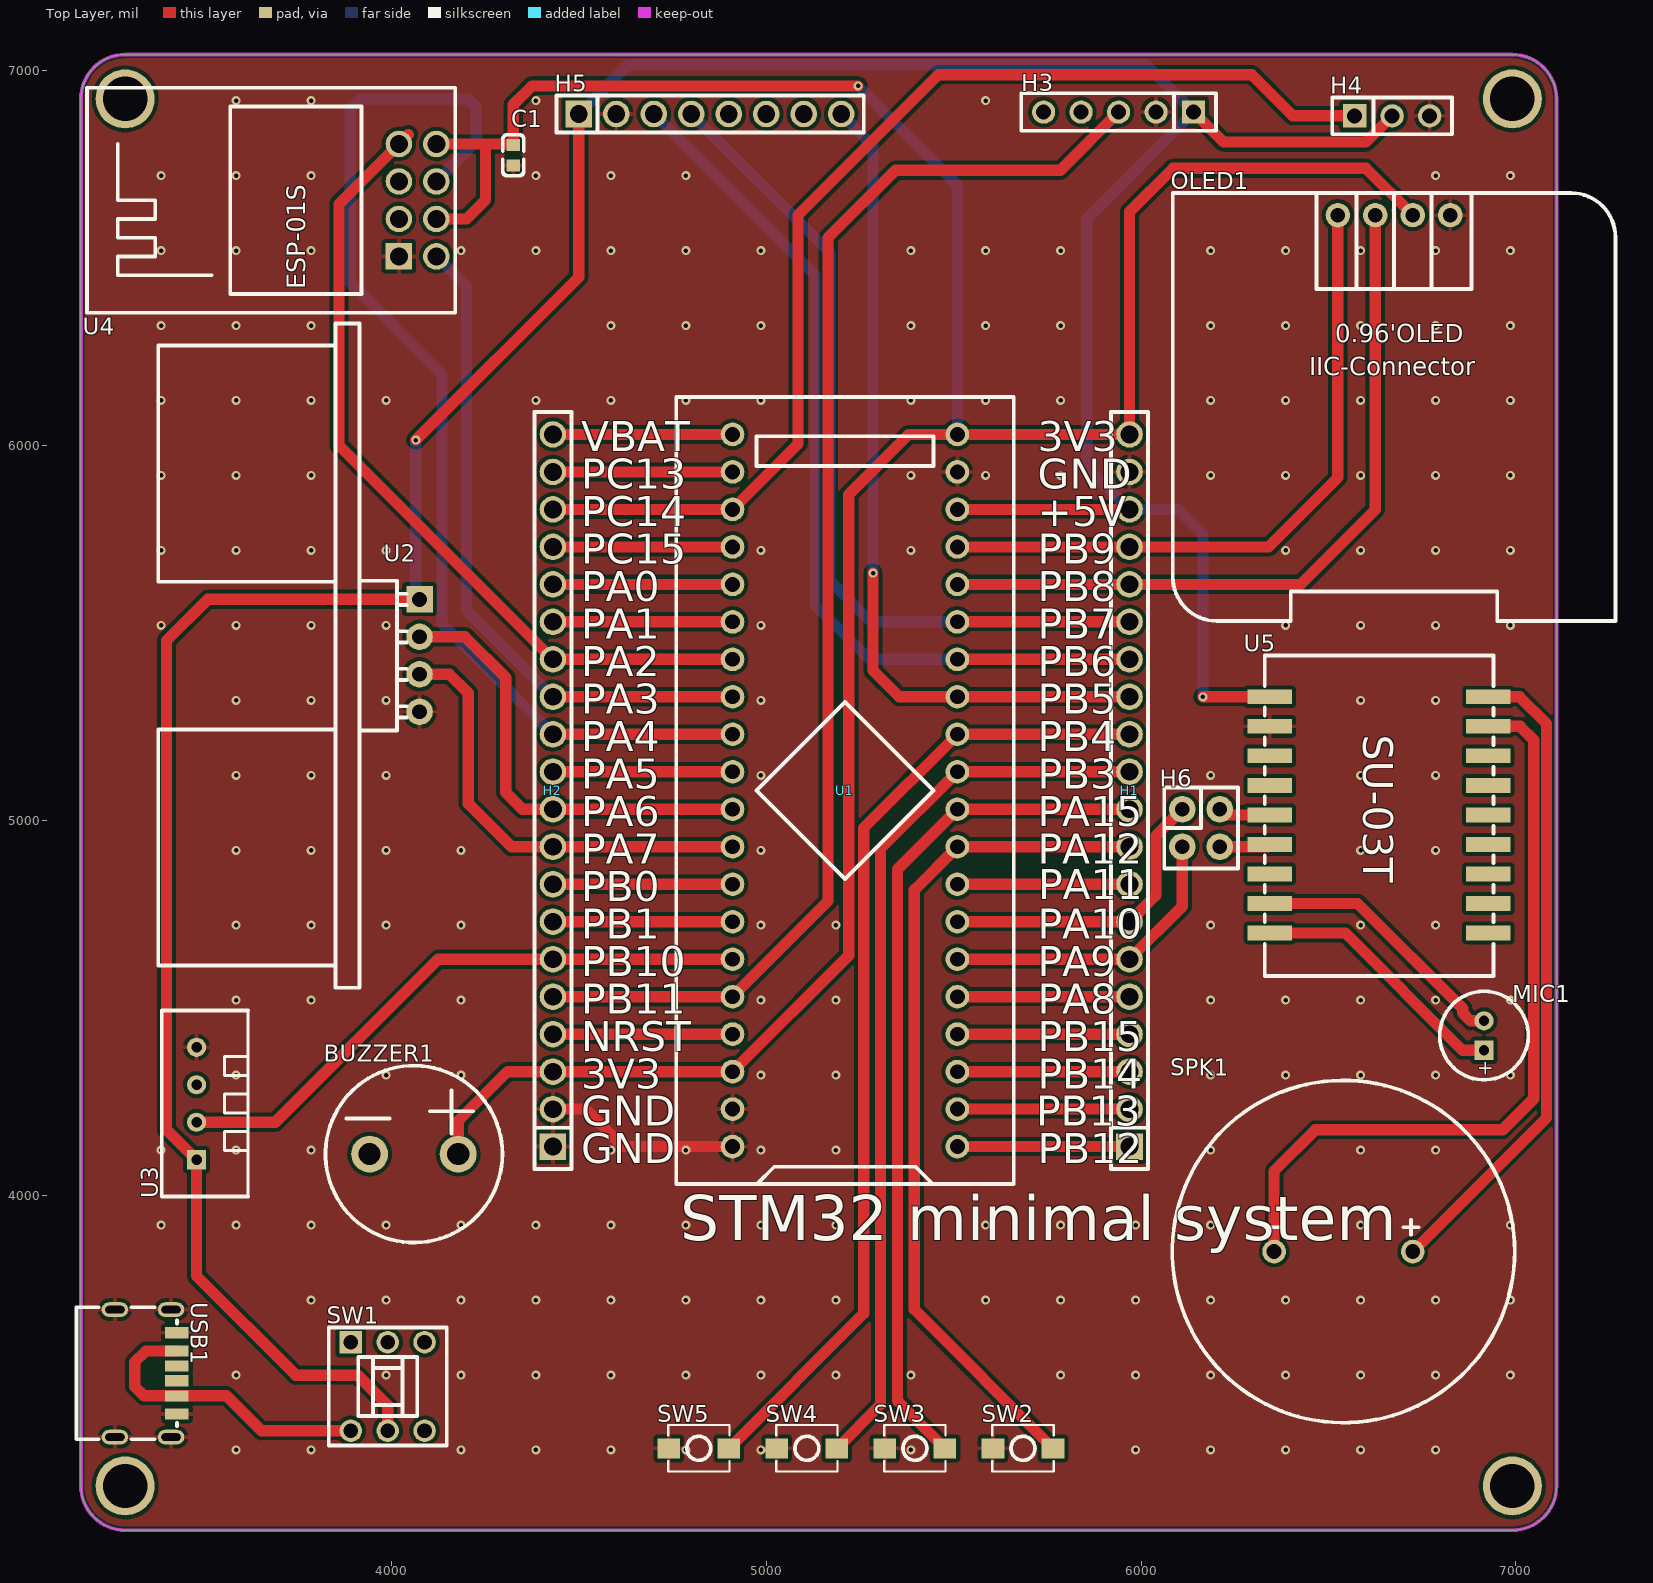
[diagram p0: Top Layer view]
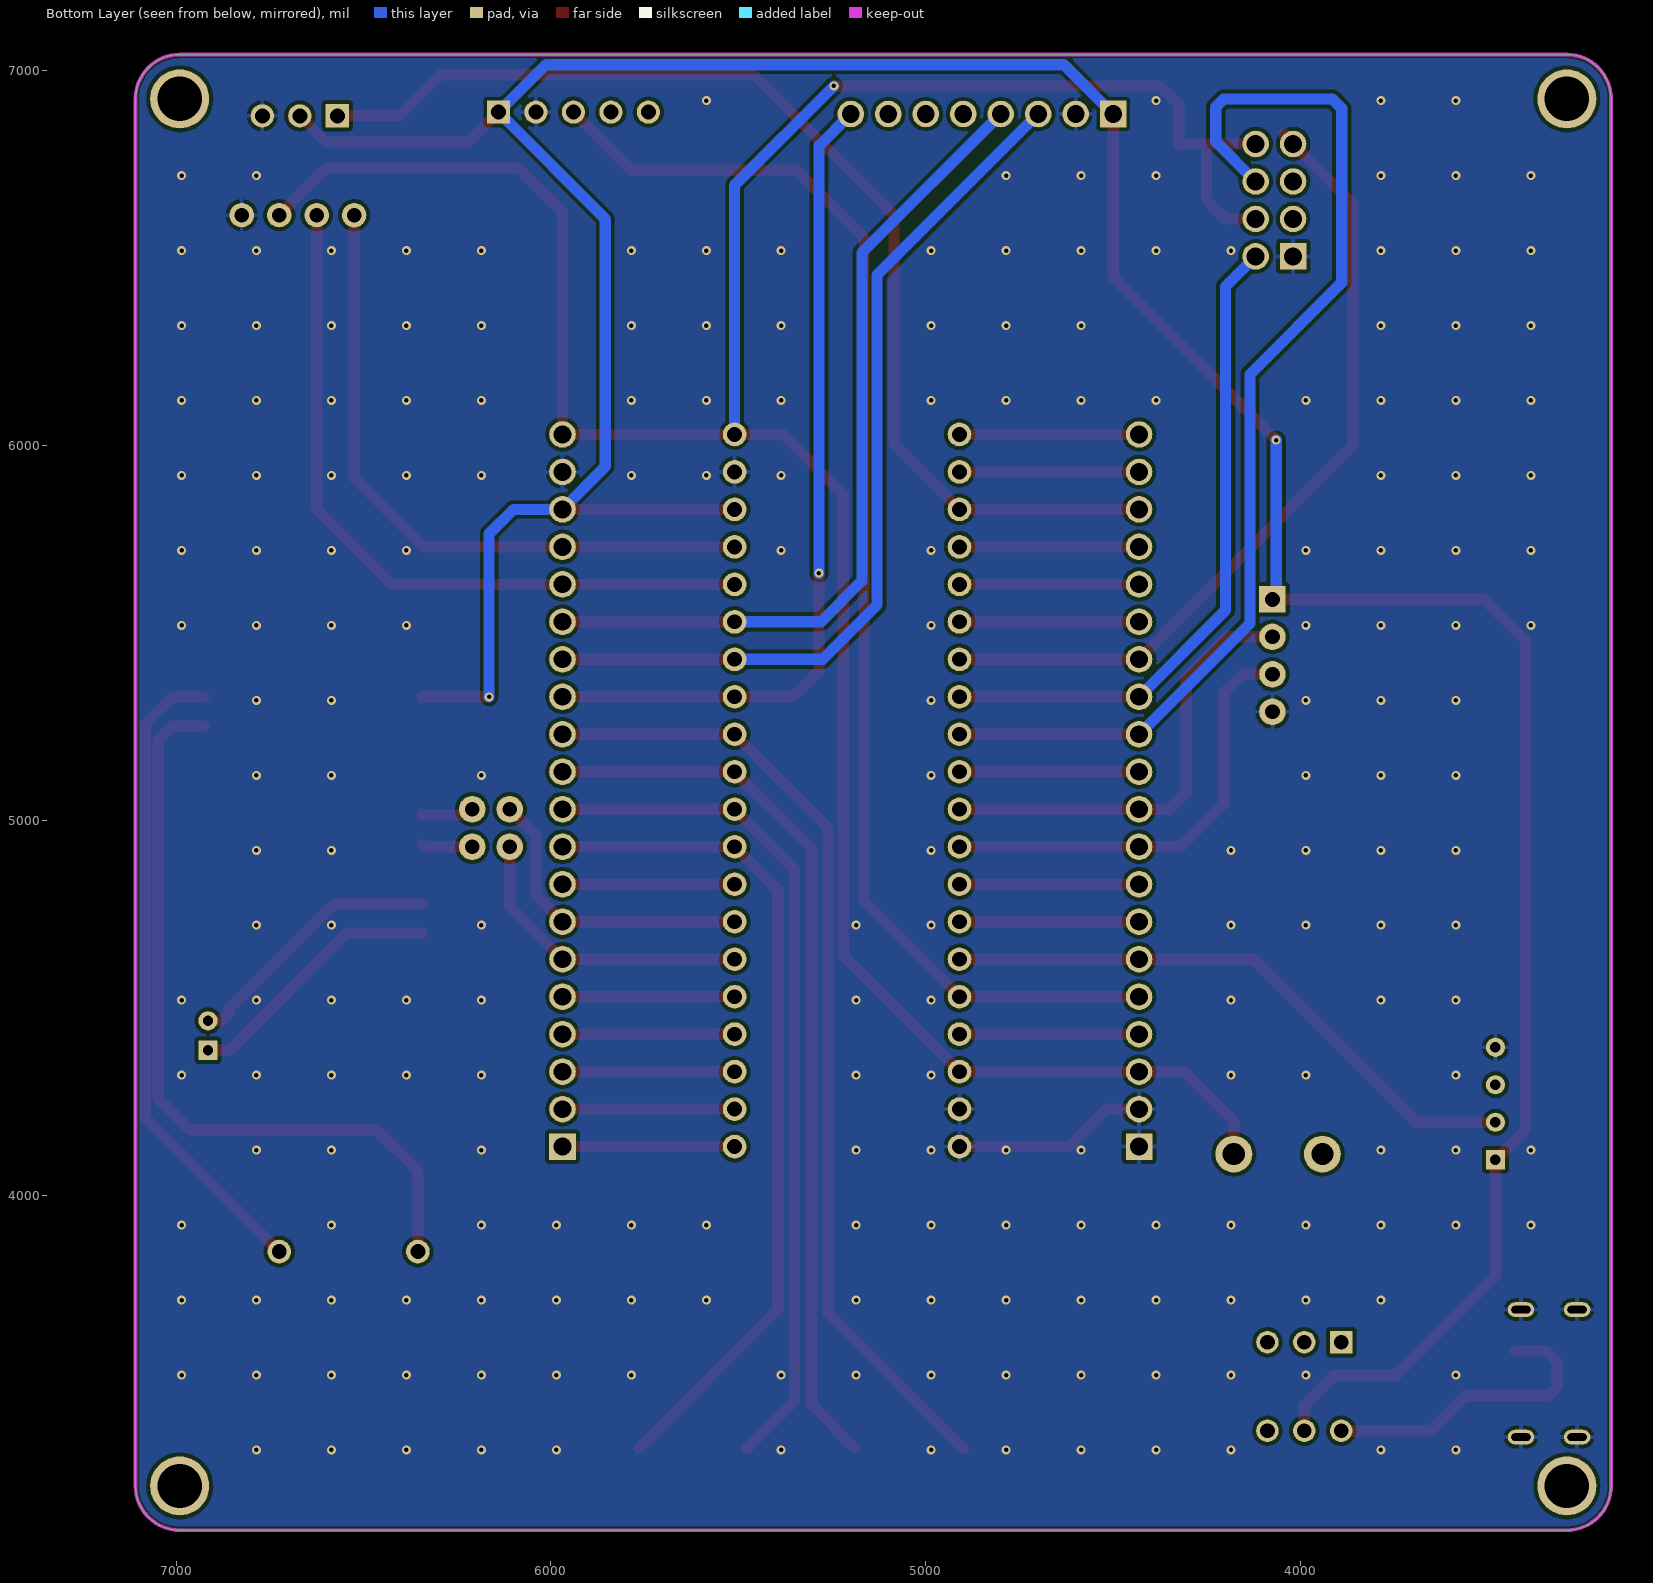
[diagram p1: Bottom Layer view, seen from below]
# Altium PCB MISC89046.pcbdoc
Units mil, origin at the board's own origin, x right, y up, seen from the top; angles counter-clockwise.
Board outline 3937.01 x 3937.01 mil, 2 copper layers (Top Layer, Bottom Layer), stack 62.206 mil thick; 22 components, 45 nets, 174 pads, 212 vias.

## Layer stack, top to bottom
Top Solder Mask Layer: solder mask 0.394, Dk 3.3
Top Layer: signal copper 1.379
Dielectric1: surface 59.449, FR4, Dk 4.5
Bottom Layer: signal copper 1.378
Bottom Solder Mask Layer: solder mask 0.394, Dk 3.3

## Board outline
3289.61,7043.5 ccw(c3289.61,6925.39) 3171.5,6925.39 3171.5,3224.61 ccw(c3289.61,3224.61) 3289.61,3106.5 6990.39,3106.5 ccw(c6990.39,3224.61) 7108.5,3224.61 7108.5,6925.39 ccw(c6990.39,6925.39) 6990.39,7043.5 3289.61,7043.5

## Design rules (kind name [scope] priority, off if disabled: settings)
BoardOutlineClearance copperThickness2oz_1 [All] p2 off: genericclearance=7.99 ignorepadtopadclearanceinfootprint=FALSE except(0: Arc-SplitContinuation Track-SplitContinuation SMDPad-SplitContinuation THPad-SplitContinuation Via-SplitContinuation Fill-SplitContinuation Region-SplitContinuation Poly-SplitContinuation Text-SplitContinuation Hole-SplitContinuation; 5.98: Arc-CutoutEdge Track-CutoutEdge SMDPad-CutoutEdge THPad-CutoutEdge Via-CutoutEdge Text-CutoutEdge; 6.9: Hole-OutlineEdge Hole-CutoutEdge; 10: Poly-OutlineEdge Poly-CutoutEdge; 11.81: Arc-OutlineEdge Track-OutlineEdge SMDPad-OutlineEdge THPad-OutlineEdge Via-OutlineEdge Fill-OutlineEdge Region-OutlineEdge Text-OutlineEdge Fill-CutoutEdge Region-CutoutEdge)
BoardOutlineClearance Plane_innerPlane_1 [All] p4 off: genericclearance=4.02 ignorepadtopadclearanceinfootprint=FALSE except(0: Arc-SplitContinuation Track-SplitContinuation SMDPad-SplitContinuation THPad-SplitContinuation Via-SplitContinuation Fill-SplitContinuation Region-SplitContinuation Poly-SplitContinuation Text-SplitContinuation Hole-SplitContinuation; 5.98: Arc-CutoutEdge Track-CutoutEdge SMDPad-CutoutEdge THPad-CutoutEdge Via-CutoutEdge Text-CutoutEdge; 6.9: Hole-OutlineEdge Hole-CutoutEdge; 10: Poly-OutlineEdge Poly-CutoutEdge; 11.81: Arc-OutlineEdge Track-OutlineEdge SMDPad-OutlineEdge THPad-OutlineEdge Via-OutlineEdge Fill-OutlineEdge Region-OutlineEdge Text-OutlineEdge Fill-CutoutEdge Region-CutoutEdge)
BoardOutlineClearance Copper_copperRegion_1 [All] p6 off: genericclearance=4.02 ignorepadtopadclearanceinfootprint=FALSE except(0: Arc-SplitContinuation Track-SplitContinuation SMDPad-SplitContinuation THPad-SplitContinuation Via-SplitContinuation Fill-SplitContinuation Region-SplitContinuation Poly-SplitContinuation Text-SplitContinuation Hole-SplitContinuation; 5.98: Arc-CutoutEdge Track-CutoutEdge SMDPad-CutoutEdge THPad-CutoutEdge Via-CutoutEdge Text-CutoutEdge; 6.9: Hole-OutlineEdge Hole-CutoutEdge; 10: Poly-OutlineEdge Poly-CutoutEdge; 11.81: Arc-OutlineEdge Track-OutlineEdge SMDPad-OutlineEdge THPad-OutlineEdge Via-OutlineEdge Fill-OutlineEdge Region-OutlineEdge Text-OutlineEdge Fill-CutoutEdge Region-CutoutEdge)
BoardOutlineClearance copperThickness1oz_1 [All] p8: genericclearance=4.02 ignorepadtopadclearanceinfootprint=FALSE except(0: Arc-SplitContinuation Track-SplitContinuation SMDPad-SplitContinuation THPad-SplitContinuation Via-SplitContinuation Fill-SplitContinuation Region-SplitContinuation Poly-SplitContinuation Text-SplitContinuation Hole-SplitContinuation; 5.98: Arc-CutoutEdge Track-CutoutEdge SMDPad-CutoutEdge THPad-CutoutEdge Via-CutoutEdge Text-CutoutEdge; 6.9: Hole-OutlineEdge Hole-CutoutEdge; 10: Poly-OutlineEdge Poly-CutoutEdge; 11.81: Arc-OutlineEdge Track-OutlineEdge SMDPad-OutlineEdge THPad-OutlineEdge Via-OutlineEdge Fill-OutlineEdge Region-OutlineEdge Text-OutlineEdge Fill-CutoutEdge Region-CutoutEdge)
Clearance copperThickness2oz [All] p1 off: gap=7.99 ignorepadtopadclearanceinfootprint=FALSE except(5.98: SMDPad-Track SMDPad-SMDPad THPad-Track SMDPad-THPad THPad-THPad Track-Via SMDPad-Via THPad-Via Via-Via Fill-SMDPad Region-SMDPad Fill-THPad Region-THPad Fill-Via Region-Via Fill-Fill Fill-Region Region-Region Arc-Track Arc-SMDPad Arc-THPad Arc-Via Fill-Arc Region-Arc Arc-Arc Text-Track SMDPad-Text Text-THPad Text-Via Fill-Text Region-Text Arc-Text Text-Text; 6.9: Hole-Track Hole-SMDPad Hole-THPad Hole-Via Fill-Hole Region-Hole Hole-Arc Hole-Text; 10: Poly-Track Poly-SMDPad Poly-THPad Poly-Via Poly-Fill Poly-Region Poly-Poly Poly-Arc Poly-Text Poly-Hole; 11.81: Fill-Track Region-Track)
Clearance Plane_innerPlane [All] p3 off: gap=4.02 ignorepadtopadclearanceinfootprint=FALSE except(5.98: SMDPad-Track SMDPad-SMDPad THPad-Track SMDPad-THPad THPad-THPad Track-Via SMDPad-Via THPad-Via Via-Via Fill-SMDPad Region-SMDPad Fill-THPad Region-THPad Fill-Via Region-Via Fill-Fill Fill-Region Region-Region Arc-Track Arc-SMDPad Arc-THPad Arc-Via Fill-Arc Region-Arc Arc-Arc Text-Track SMDPad-Text Text-THPad Text-Via Fill-Text Region-Text Arc-Text Text-Text; 6.9: Hole-Track Hole-SMDPad Hole-THPad Hole-Via Fill-Hole Region-Hole Hole-Arc Hole-Text; 10: Poly-Track Poly-SMDPad Poly-THPad Poly-Via Poly-Fill Poly-Region Poly-Poly Poly-Arc Poly-Text Poly-Hole; 11.81: Fill-Track Region-Track)
Clearance Copper_copperRegion [All] p5 off: gap=4.02 ignorepadtopadclearanceinfootprint=FALSE except(5.98: SMDPad-Track SMDPad-SMDPad THPad-Track SMDPad-THPad THPad-THPad Track-Via SMDPad-Via THPad-Via Via-Via Fill-SMDPad Region-SMDPad Fill-THPad Region-THPad Fill-Via Region-Via Fill-Fill Fill-Region Region-Region Arc-Track Arc-SMDPad Arc-THPad Arc-Via Fill-Arc Region-Arc Arc-Arc Text-Track SMDPad-Text Text-THPad Text-Via Fill-Text Region-Text Arc-Text Text-Text; 6.9: Hole-Track Hole-SMDPad Hole-THPad Hole-Via Fill-Hole Region-Hole Hole-Arc Hole-Text; 10: Poly-Track Poly-SMDPad Poly-THPad Poly-Via Poly-Fill Poly-Region Poly-Poly Poly-Arc Poly-Text Poly-Hole; 11.81: Fill-Track Region-Track)
Clearance copperThickness1oz [All] p7: gap=4.02 ignorepadtopadclearanceinfootprint=FALSE except(5.98: SMDPad-Track SMDPad-SMDPad THPad-Track SMDPad-THPad THPad-THPad Track-Via SMDPad-Via THPad-Via Via-Via Fill-SMDPad Region-SMDPad Fill-THPad Region-THPad Fill-Via Region-Via Fill-Fill Fill-Region Region-Region Arc-Track Arc-SMDPad Arc-THPad Arc-Via Fill-Arc Region-Arc Arc-Arc Text-Track SMDPad-Text Text-THPad Text-Via Fill-Text Region-Text Arc-Text Text-Text; 6.9: Hole-Track Hole-SMDPad Hole-THPad Hole-Via Fill-Hole Region-Hole Hole-Arc Hole-Text; 10: Poly-Track Poly-SMDPad Poly-THPad Poly-Via Poly-Fill Poly-Region Poly-Poly Poly-Arc Poly-Text Poly-Hole; 11.81: Fill-Track Region-Track)
DiffPairsRouting differentialPair [All] p1: maxlimit=6 minlimit=6 mostfreqgap=6 toplayer_minwidth=5 toplayer_prefwidth=10 toplayer_maxwidth=100 toplayer_mingap=6 toplayer_prefgap=6 toplayer_maxgap=6 bottomlayer_minwidth=5 bottomlayer_prefwidth=10 bottomlayer_maxwidth=100 bottomlayer_mingap=6 bottomlayer_prefgap=6 bottomlayer_maxgap=6 maxuncoupledlength=10
HoleToHoleClearance otherClearance [All] p1: gap=11.81 allowstackedmicrovias=TRUE
Length netLength [All] p1: minlimit=0 maxlimit=0
PasteMaskExpansion pasteMaskExpansion [All] p1: expansion=0
PlaneConnect innerPlane [All] p1: planeconnectstyle=Relief reliefexpansion=20 reliefentries=4 reliefconductorwidth=10 reliefairgap=10
PolygonConnect copperRegion [All] p1: connectstyle=Relief reliefconductorwidth=10 reliefentries=4 polygonreliefangle="90 Angle" airgapwidth=10 via.connectstyle=Relief via.reliefconductorwidth=10 via.reliefentries=4 via.polygonreliefangle="90 Angle" via.airgapwidth=10
RoutingVias viaSize [All] p1: holewidth=12.01 width=24.02 viastyle="Through Hole" minholewidth=11.81 minwidth=19.68 maxholewidth=248.03 maxwidth=393.7
SolderMaskExpansion solderMaskExpansion [IsVia] p1: expansion=-1000 istentingtop=TRUE
SolderMaskExpansion solderMaskExpansion [All] p2: expansion=2 istentingtop=FALSE
Width copperThickness2oz_2 [All] p1 off: maxlimit=100 minlimit=8 preferedwidth=10
Width copperThickness1oz_2 [All] p2: maxlimit=100 minlimit=5 preferedwidth=10

## Components (designator, comment, footprint, x,y, rotation, side; value= is the part's Value field where it differs from the comment)
BUZZER1 "Buz" BUZ-TH_BD12.0-P6.00-D0.9-RD 4060,4110 r0 top
C1 "100nF" C0603 4325,6775 r270 top
H1 "" HDR-TH_20P-P2.54-V-F 5969.16,5080 r90 top
H2 "" HDR-TH_20P-P2.54-V-F 4430.95,5080 r90 top
H3 "ATGM336H module" HDR-TH_5P-P2.54-V-F 5940,6890 r180 top
H4 "Vibration module" HDR-TH_3P-P2.54-V-F 6670,6880 r0 top
H5 "MPU6050" HDR-TH_8P-P2.54-V-F-1 4850,6885 r0 top
H6 "" HDR-TH_4P-P2.54-V-F-R2-C2-S2.54 6160,4980 r270 top
MIC1 "MIC" MIC-TH_BD6.0-P2.00 6915,4426.26 r90 top
OLED1 "" 0.96OLED_4P 6675,6615 r0 top
SPK1 "FS-2308" BEEP-TH_BD23.2-P9.20-D1.0 6540,3850 r0 top
SW1 "PS081-06L135D1-JF-G" SW-TH_6P-L8.0-W8.0-P2.50-TL 3990,3490 r0 top
SW2 "" Key_SMD_3x4x2 5685,3325 r0 top
SW3 "" Key_SMD_3x4x2 5396.67,3325 r0 top
SW4 "" Key_SMD_3x4x2 5108.33,3325 r0 top
SW5 "" Key_SMD_3x4x2 4820,3325 r0 top
U1 "STM32F103C8T6-Card" CONN-TH_L53.3-W22.9_STM32F103C8T6-CARD 5210,5080 r90 top
U2 "HC-SR04" TH_HC-SR04V 4075,5440 r270 top
U3 "DHT11 temperature and humidity" SENSOR-TH_DHT11 3480,4245 r90 top
U4 "ESP-01S" WIFIM-TH_ESP-01S 4070,6655 r90 top
U5 "SU-03T" COMM-SMD_18P-L21.0-W15.0-P2.00 6635,5015 r0 top
USB1 "TYPEC-250D-BCP6" USB-C-SMD_TYPEC-250D-BCP6 3345,3525 r270 top

## Footprints (in the part's own frame and the unit in brackets; to place one, negate y for a bottom-side part, rotate by r counter-clockwise, add the part's x,y. Pads: shape width x height; smd on the part's side, far side on the other; paste and mask are expansions set on the pad)
0.96OLED_4P [mm]
  round 1.65 hole 1 copper offset 0,0: 1(-3.81,-0.001) 2(-1.27,0.002) 3(1.27,0.002) 4(3.81,0.002)
  silkscreen extent -15,-27.5 15,1.5
BEEP-TH_BD23.2-P9.20-D1.0 [mm]
  round 1.6 hole 1: 1(4.7,0) 2(-4.7,0)
  silkscreen extent -11.6,-11.6 11.6,11.6
BUZ-TH_BD12.0-P6.00-D0.9-RD [mm]
  round 2.5 hole 1.5 paste+0 mask+0.05: 1(-3,0) 2(3,0)
  silkscreen extent -5.99,-5.99 5.99,5.99
C0603 [mm]
  rect 0.8x0.9 smd: 1(-0.7,0) 2(0.7,0)
  silkscreen extent -1.39,-0.71 1.39,0.71
COMM-SMD_18P-L21.0-W15.0-P2.00 [mm]
  rect 3x1 smd: 1(-7.4,8) 2(-7.4,6) 3(-7.4,4) 4(-7.4,2) 5(-7.4,0) 6(-7.4,-2) 7(-7.4,-4) 8(-7.4,-6) 9(-7.4,-8) 10(7.4,-8) 11(7.4,-6) 12(7.4,-4) 13(7.4,-2) 14(7.4,0) 15(7.4,2) 16(7.4,4) 17(7.4,6) 18(7.4,8)
  silkscreen extent -7.75,-10.92 7.75,10.79
CONN-TH_L53.3-W22.9_STM32F103C8T6-CARD [mm]
  round 1.6 hole 1: 1(-24.13,-7.62) 2(-21.59,-7.62) 3(-19.05,-7.62) 4(-16.51,-7.62) 5(-13.97,-7.62) 6(-11.43,-7.62) 7(-8.89,-7.62) 8(-6.35,-7.62) 9(-3.81,-7.62) 10(-1.27,-7.62) 11(1.27,-7.62) 12(3.81,-7.62) 13(6.35,-7.62) 14(8.89,-7.62) 15(11.43,-7.62) 16(13.97,-7.62) 17(16.51,-7.62) 18(19.05,-7.62) 19(21.59,-7.62) 20(24.13,-7.62) 21(24.13,7.62) 22(21.59,7.62) 23(19.05,7.62) 24(16.51,7.62) 25(13.97,7.62) 26(11.43,7.62) 27(8.89,7.62) 28(6.35,7.62) 29(3.81,7.62) 30(1.27,7.62) 31(-1.27,7.62) 32(-3.81,7.62) 33(-6.35,7.62) 34(-8.89,7.62) 35(-11.43,7.62) 36(-13.97,7.62) 37(-16.51,7.62) 38(-19.05,7.62) 39(-21.59,7.62) 40(-24.13,7.62)
  silkscreen extent -26.67,-11.43 26.67,11.43
HDR-TH_3P-P2.54-V-F [mil]
  rect 62x62 hole 40.16: 1(-100,0)
  round 62 hole 40.16: 2(0,0) 3(100,0)
  silkscreen extent -160,-49 160,49
HDR-TH_4P-P2.54-V-F-R2-C2-S2.54 [mm]
  round 1.8 hole 1: 1(-1.27,-1.27) 2(-1.27,1.27) 3(1.27,-1.27) 4(1.27,1.27)
  silkscreen extent -2.74,-2.5 2.74,2.5
HDR-TH_5P-P2.54-V-F [mil]
  rect 62x62 hole 40.16: 1(-200,0)
  round 62 hole 40.16: 2(-100,0) 3(0,0) 4(100,0) 5(200,0)
  silkscreen extent -260,-50 260,50
HDR-TH_8P-P2.54-V-F-1 [mm]
  rect 1.8x1.8 hole 1.2: 1(-8.89,0)
  round 1.8 hole 1.2: 2(-6.35,0) 3(-3.81,0) 4(-1.27,0) 5(1.27,0) 6(3.81,0) 7(6.35,0) 8(8.89,0)
  silkscreen extent -10.41,-1.25 10.41,1.25
HDR-TH_20P-P2.54-V-F [mm]
  rect 1.8x1.8 hole 1.2: 1(-24.13,0)
  round 1.8 hole 1.2: 2(-21.59,0) 3(-19.05,0) 4(-16.51,0) 5(-13.97,0) 6(-11.43,0) 7(-8.89,0) 8(-6.35,0) 9(-3.81,0) 10(-1.27,0) 11(1.27,0) 12(3.81,0) 13(6.35,0) 14(8.89,0) 15(11.43,0) 16(13.97,0) 17(16.51,0) 18(19.05,0) 19(21.59,0) 20(24.13,0)
  silkscreen extent -25.65,-1.25 25.65,1.25
Key_SMD_3x4x2 [mm]
  rect 1.53x1.36 smd paste+0 mask+0.051: 1(-2.035,0) 2(2.035,0)
  silkscreen extent -2.08,-1.58 2.08,1.58
MIC-TH_BD6.0-P2.00 [mm]
  rect 1.3x1.3 hole 0.7: 1(-1,0)
  round 1.3 hole 0.7: 2(1,0)
  silkscreen extent -3,-3 3,3
SENSOR-TH_DHT11 [mil]
  rect 51x51 hole 28: 1(-150,0)
  round 51 hole 28: 2(-50,0) 3(50,0) 4(150,0)
  silkscreen extent -248,-138 248,93
SW-TH_6P-L8.0-W8.0-P2.50-TL [mil]
  rect 60x60 hole 39.37: 1(-98.43,118.11)
  round 60 hole 39.37: 2(0,118.11) 3(98.42,118.11) 4(-98.43,-118.11) 5(0,-118.11) 6(98.42,-118.11)
  silkscreen extent -157,-157 157,157
TH_HC-SR04V [mm]
  rect 1.8x1.8 hole 1.001: 1(-3.81,0)
  round 1.8 hole 1.001: 2(-1.27,0) 3(1.27,0) 4(3.81,0)
  silkscreen extent -22.5,-17.7 22.5,-0.89
USB-C-SMD_TYPEC-250D-BCP6 [mm]
  oval 1x1.8 hole 0.5 slot 1.3 at 90 deg paste+0 mask+0.05: 1(-4.32,1.7) 2(-4.32,-2.1) 3(4.32,-2.1) 4(4.32,1.7)
  rect 0.75x1.6 smd paste-100 mask+0.05: A5(-0.5,2.1) A9(1.52,2.1) B5(0.5,2.1) B9(-1.52,2.1)
  rect 0.75x1.6 smd paste-100 mask+0.051: A12(2.75,2.1) B12(-2.75,2.1)
  silkscreen extent -4.48,-4.7 4.47,2.1
WIFIM-TH_ESP-01S [mm]
  rect 1.8x1.8 hole 1.2: 1(-3.81,1.27)
  round 1.8 hole 1.2: 2(-1.27,1.27) 3(1.27,1.27) 4(3.81,1.27) 5(3.81,-1.27) 6(1.27,-1.27) 7(-1.27,-1.27) 8(-3.81,-1.27)
  silkscreen extent -7.62,-2.54 7.62,22.4

## Free pads (board coordinates)
  round 157.48 hole 118.11: 1(3289.61,6925.39) 1(3289.61,3224.61) 1(6990.39,6925.39) 1(6990.39,3224.61)

## Via types
v1: diameter 24.02, hole 12, Top Layer to Bottom Layer, 212 vias

## Nets (pads, with @x,y where several pads share a name; then routed paths per layer and width w, separated by ;. In a path a pad name is that pad's centre, name@x,y a point inside that pad or via, vN(x,y) a via of type N, cw(c..) or ccw(c..) an arc to the next point about the centre after c; other vN are vias at no path point)
$1N17032: MIC1.1 U5.9 | length 701
  Top Layer w30: U5.9 6544.97,4700.03 6858.11,4386.89 MIC1.1
$1N17033: MIC1.2 U5.8 | length 707.7
  Top Layer w30: U5.8 6577.59,4778.77 6858.2,4498.16 6858.2,4486.84 6879.41,4465.63 MIC1.2
$1N17034: SPK1.1 U5.18 | length 1741.1
  Top Layer w30: SPK1.1 7081.69,4206.65 7081.69,5258.31 7010.04,5329.96 U5.18
$1N17035: SPK1.2 U5.17 | length 2081.2
  Top Layer w30: SPK1.2 6354.96,4064.96 6465,4175 6965,4175 7047.68,4257.68 7047.68,5215 7011.46,5251.22 U5.17
$1N17038: H6.2 U5.5 | length 139.9
  Top Layer w30: H6.2 6225,5015 U5.5
$1N17039: H6.4 U5.6 | length 136.2
  Top Layer w30: H6.4 6337.41,4930 U5.6
+3V3: BUZZER1.2 C1.1 H1.20 H2.3 OLED1.3 U1.20 U1.38 U4.5 U4.7 | length 7403.2
  Top Layer w30: U4.7 4200,6605 4250.83,6655.83 4250.83,6805 ; U4.5 4250.83,6805 ; BUZZER1.2 4178.11,4198.11 4310,4330 H2.3 U1.38 5220,4640 5220,5870 5380,6030 U1.20 H1.20 5969.16,6624.16 6085,6740 6600.05,6740 OLED1.3@6725,6615.05 ; v1(5245,6960) 4375,6960 4325,6910 C1.1 4322.56,6805 4250.83,6805
  Bottom Layer w30: v1(5245,6960) 5510,6695 U1.20
+5V: H1.18 H3.1 H4.2 H5.1 SW1.5 U1.18 U2.1 U3.1 U5.1 | length 9509.1
  Top Layer w30: SW1.5 3990.01,3439.99 3910,3520 3745,3520 3480,3785 U3.1 3400,4175 3400,5480 3510,5590 U2.1 ; v1(4065,6015) 4500,6450 H5.1 ; U1.18 H1.18 ; H3.1 6220,6810 6600,6810 H4.2 ; v1(6165,5330) U5.1@6343.63,5330
  Bottom Layer w30: v1(4065,6015) 4065,5600 U2.1 ; H5.1 4631.69,7016.69 6013.31,7016.69 H3.1 5855,6605 5855,5944.16 H1.18 6100,5830 6165,5765 v1(6165,5330)
GND: C1.2 H1.19 H2.1 H2.2 H3.2 H4.3 H5.2 OLED1.4 SW2.1 SW3.1 SW4.1 SW5.1 U1.19 U1.39 U1.40 U2.4 U3.4 U4.1 U5.2 USB1.1 USB1.2 USB1.3 USB1.4 USB1.A12 USB1.B12 | length 520.5
  Top Layer w30: H2.2 4517.8,4230 4617.8,4130 U1.40
  other v1: 3585.6,3320.6 3785.6,3320.6 4185.6,3320.6 4385.6,3320.6 4585.6,3320.6 4785.6,3320.6 4985.6,3320.6 5385.6,3320.6 5985.6,3320.6 6185.6,3320.6 6385.6,3320.6 6585.6,3320.6 6785.6,3320.6 3585.6,3520.6 3985.6,3520.6 4185.6,3520.6 4385.6,3520.6 4585.6,3520.6 4785.6,3520.6 4985.6,3520.6 5185.6,3520.6 5385.6,3520.6 5785.6,3520.6 5985.6,3520.6 6185.6,3520.6 6385.6,3520.6 6585.6,3520.6 6785.6,3520.6 6985.6,3520.6 3785.6,3720.6 3985.6,3720.6 4185.6,3720.6 4385.6,3720.6 4585.6,3720.6 4785.6,3720.6 4985.6,3720.6 5185.6,3720.6 5585.6,3720.6 5785.6,3720.6 5985.6,3720.6 6185.6,3720.6 6385.6,3720.6 6585.6,3720.6 6785.6,3720.6 6985.6,3720.6 3385.6,3920.6 3585.6,3920.6 3785.6,3920.6 3985.6,3920.6 4185.6,3920.6 4385.6,3920.6 4585.6,3920.6 4785.6,3920.6 4985.6,3920.6 5185.6,3920.6 5585.6,3920.6 5785.6,3920.6 5985.6,3920.6 6185.6,3920.6 6585.6,3920.6 6985.6,3920.6 3385.6,4120.6 3585.6,4120.6 3785.6,4120.6 4585.6,4120.6 4785.6,4120.6 4985.6,4120.6 5185.6,4120.6 6185.6,4120.6 6585.6,4120.6 6785.6,4120.6 3585.6,4320.6 3985.6,4320.6 4185.6,4320.6 4985.6,4320.6 5185.6,4320.6 6185.6,4320.6 6385.6,4320.6 6585.6,4320.6 6785.6,4320.6 6985.6,4320.6 3585.6,4520.6 3785.6,4520.6 4185.6,4520.6 4985.6,4520.6 5185.6,4520.6 6185.6,4520.6 6385.6,4520.6 6585.6,4520.6 6785.6,4520.6 6985.6,4520.6 3585.6,4720.6 3785.6,4720.6 3985.6,4720.6 4185.6,4720.6 4985.6,4720.6 5185.6,4720.6 6185.6,4720.6 6585.6,4720.6 6785.6,4720.6 3585.6,4920.6 3785.6,4920.6 3985.6,4920.6 4185.6,4920.6 4985.6,4920.6 6585.6,4920.6 6785.6,4920.6 3585.6,5120.6 3785.6,5120.6 3985.6,5120.6 4985.6,5120.6 6185.6,5120.6 6585.6,5120.6 6785.6,5120.6 3585.6,5320.6 3785.6,5320.6 3985.6,5320.6 4985.6,5320.6 6585.6,5320.6 6785.6,5320.6 3385.6,5520.6 3585.6,5520.6 3785.6,5520.6 3985.6,5520.6 4985.6,5520.6 6385.6,5520.6 6585.6,5520.6 6785.6,5520.6 6985.6,5520.6 3385.6,5720.6 3585.6,5720.6 3785.6,5720.6 3985.6,5720.6 4985.6,5720.6 5385.6,5720.6 6385.6,5720.6 6585.6,5720.6 6785.6,5720.6 6985.6,5720.6 3385.6,5920.6 3585.6,5920.6 3785.6,5920.6 5385.6,5920.6 5585.6,5920.6 5785.6,5920.6 6185.6,5920.6 6385.6,5920.6 6585.6,5920.6 6785.6,5920.6 6985.6,5920.6 3385.6,6120.6 3585.6,6120.6 3785.6,6120.6 3985.6,6120.6 4385.6,6120.6 4585.6,6120.6 4785.6,6120.6 4985.6,6120.6 5385.6,6120.6 5585.6,6120.6 5785.6,6120.6 6185.6,6120.6 6385.6,6120.6 6585.6,6120.6 6785.6,6120.6 6985.6,6120.6 3385.6,6320.6 3585.6,6320.6 3785.6,6320.6 4585.6,6320.6 4785.6,6320.6 4985.6,6320.6 5385.6,6320.6 5585.6,6320.6 5785.6,6320.6 6185.6,6320.6 6385.6,6320.6 6585.6,6320.6 6785.6,6320.6 6985.6,6320.6 3385.6,6520.6 3585.6,6520.6 3785.6,6520.6 4185.6,6520.6 4385.6,6520.6 4585.6,6520.6 4785.6,6520.6 4985.6,6520.6 5385.6,6520.6 5585.6,6520.6 5785.6,6520.6 6185.6,6520.6 6385.6,6520.6 6585.6,6520.6 6785.6,6520.6 6985.6,6520.6 3385.6,6720.6 3585.6,6720.6 3785.6,6720.6 4385.6,6720.6 4585.6,6720.6 4785.6,6720.6 6785.6,6720.6 6985.6,6720.6 3585.6,6920.6 3785.6,6920.6 4385.6,6920.6 5585.6,6920.6
NET13: BUZZER1.1
PA0: H2.16 U1.25 | length 479
  Top Layer w30: H2.16 U1.25
PA1: H2.15 U1.26 | length 479
  Top Layer w30: H2.15 U1.26
PA2_TX: H2.14 U1.27 U4.4 | length 2192.2
  Top Layer w30: U4.4@4045,6830 3860,6645 3860,6000.95 H2.14 U1.27
PA3_RX: H2.13 U1.28 U4.8 | length 1782.8
  Top Layer w30: H2.13 U1.28
  Bottom Layer w30: U4.8 4200,6425 4200,5560.95 H2.13
PA4_WIFIRST: H2.12 U1.29 U4.6 | length 2971.3
  Top Layer w30: H2.12 U1.29
  Bottom Layer w30: U4.6 4226.21,6811.21 4226.21,6903.79 4205,6925 3915,6925 3890,6900 3890,6435 4135,6190 4135,5525.95 H2.12
PA5: H2.11 U1.30 | length 479
  Top Layer w30: H2.11 U1.30
PA6_TRIG2: H2.10 U1.31 U2.2 | length 1205
  Top Layer w30: U2.2 4196.42,5490 4305,5381.42 4305,5075 4350,5030 H2.10 U1.31
PA7_ECHO2: H2.9 U1.32 U2.3 | length 1198.3
  Top Layer w30: U2.3 4155,5390 4205,5340 4205,5045 4320,4930 H2.9 U1.32
PA8: H1.5 U1.5 | length 459.2
  Top Layer w30: U1.5 H1.5
PA9_TX: H1.6 H6.3 U1.6 | length 817.5
  Top Layer w30: U1.6 H1.6 6110,4770.84 H6.3
PA10_RX: H1.7 H6.1 U1.7 | length 817.5
  Top Layer w30: U1.7 H1.7 6040,4800.84 6040,4960 H6.1
PA11: H1.8 U1.8 | length 459.2
  Top Layer w30: U1.8 H1.8
PA12_KEY1: H1.9 SW2.2 U1.9 | length 2265.1
  Top Layer w30: SW2.2 5395,3695.12 5395,4815 U1.9 H1.9
PA15_KEY2: H1.10 SW3.2 U1.10 | length 2283
  Top Layer w30: SW3.2 5350,3451.79 5350,4870 U1.10 H1.10
PB0: H2.8 U1.33 | length 479
  Top Layer w30: H2.8 U1.33
PB1: H2.7 U1.34 | length 479
  Top Layer w30: H2.7 U1.34
PB3_KEY3: H1.11 SW4.2 U1.11 | length 2397.3
  Top Layer w30: SW4.2 5305,3441.55 5305,4925 U1.11 H1.11
PB4_KEY4: H1.12 SW5.2 U1.12 | length 2616.8
  Top Layer w30: SW5.2 5260,3684.88 5260,4980 U1.12 H1.12
PB5_MPUINT: H1.13 H5.8 U1.13 | length 2233.4
  Top Layer w30: v1(5285,5660) 5285,5400 5355,5330 U1.13 H1.13
  Bottom Layer w30: H5.8 5285,6800 v1(5285,5660)
PB6_MPUSCL: H1.14 H5.3 U1.14 | length 2387.3
  Top Layer w30: U1.14 H1.14
  Bottom Layer w30: H5.3 5130,6455 5130,5575 5275,5430 U1.14
PB7_MPUSDA: H1.15 H5.4 U1.15 | length 2243
  Top Layer w30: U1.15 H1.15
  Bottom Layer w30: H5.4 5170,6515 5170,5640 5280,5530 U1.15
PB8_OLEDSCL: H1.16 OLED1.2 U1.16 | length 1982.9
  Top Layer w30: U1.16 H1.16 6425,5630 6625,5830 OLED1.2@6625,6615.05
PB9_OLEDSDA: H1.17 OLED1.1 U1.17 | length 1791.6
  Top Layer w30: U1.17 H1.17 6340,5730 6525,5915 OLED1.1
PB10_DHT11: H2.6 U1.35 U3.2 | length 1610.2
  Top Layer w30: U3.2 3690,4195 4125,4630 H2.6 U1.35
PB11_GPSTX: H2.5 H3.3 U1.36 | length 3523.4
  Top Layer w30: H2.5 U1.36 5165,4785 5165,6555 5345,6735 5785,6735 H3.3
PB12: H1.1 U1.1 | length 459.2
  Top Layer w30: U1.1 H1.1
PB13: H1.2 U1.2 | length 459.2
  Top Layer w30: U1.2 H1.2
PB14: H1.3 U1.3 | length 459.2
  Top Layer w30: U1.3 H1.3
PB15: H1.4 U1.4 | length 459.2
  Top Layer w30: U1.4 H1.4
PC13_BEEP: H2.19 U1.22 | length 479
  Top Layer w30: H2.19 U1.22
PC14_VIBRATE: H2.18 H4.1 U1.23 | length 3022.4
  Top Layer w30: H2.18 U1.23 5085,6005 5085,6615 5460,6990 6295,6990 6405,6880 H4.1
PC15: H2.17 U1.24 | length 479
  Top Layer w30: H2.17 U1.24
RST: H2.4 U1.37 | length 479
  Top Layer w30: H2.4 U1.37
VBAT: H2.20 U1.21 | length 479
  Top Layer w30: H2.20 U1.21
VBUS: SW1.4 USB1.A9 USB1.B9 | length 815.5
  Top Layer w30: USB1.B9 3344.85,3584.85 3315,3555 3315,3490 3339.84,3465.16 USB1.A9 3559.84,3465.16 3653.11,3371.89 SW1.4
pads on no net: H3.4 H3.5 H5.5 H5.6 H5.7 SW1.1 SW1.2 SW1.3 SW1.6 U3.3 U4.2 U4.3 U5.3 U5.4 U5.7 U5.10 U5.11 U5.12 U5.13 U5.14 U5.15 U5.16 USB1.A5 USB1.B5

## Polygon pours and split planes (outlines as drawn)
GND on Bottom Layer (solid, remove dead copper, pour order 2): 3100,7165 3100,3000 7275,3000 7275,7165
GND on Top Layer (solid, remove dead copper, pour order 0): 3000,7145 3000,3075 7385,3075 7385,7145

## Keep-outs
Board Outline Layer:
  the board outline again, w10

## Silkscreen, mask and mechanical layers (free items; w line width, h text height)
Top Silkscreen Layer:
  text "VBAT" at 4505.95,5985 h80
  text "3V3" at 5724.16,5985 h80
  text "PC13" at 4505.95,5885 h80
  text "GND" at 5724.16,5885 h80
  text "PC14" at 4505.95,5785 h80
  text "+5V" at 5724.16,5785 h80
  text "PC15" at 4505.95,5685 h80
  text "PB9" at 5724.16,5685 h80
  text "PA0" at 4505.95,5585 h80
  text "PB8" at 5724.16,5585 h80
  text "PA1" at 4505.95,5485 h80
  text "PB7" at 5724.16,5485 h80
  text "PA2" at 4505.95,5385 h80
  text "PB6" at 5724.16,5385 h80
  text "PA3" at 4505.95,5285 h80
  text "PB5" at 5724.16,5285 h80
  text "PA4" at 4505.95,5185 h80
  text "PB4" at 5724.16,5185 h80
  text "PA5" at 4505.95,5085 h80
  text "PB3" at 5724.16,5085 h80
  text "PA6" at 4505.95,4985 h80
  text "PA15" at 5724.16,4985 h80
  text "PA7" at 4505.95,4885 h80
  text "PA12" at 5724.16,4885 h80
  text "PA11" at 5725.95,4790 h80
  text "PB0" at 4505.95,4785 h80
  text "PB1" at 4505.95,4685 h80
  text "PA10" at 5724.16,4685 h80
  text "PB10" at 4505.95,4585 h80
  text "PA9" at 5724.16,4585 h80
  text "PB11" at 4505.95,4485 h80
  text "PA8" at 5724.16,4485 h80
  text "NRST" at 4505.95,4385 h80
  text "PB15" at 5724.16,4385 h80
  text "3V3" at 4505.95,4285 h80
  text "PB14" at 5724.16,4285 h80
  text "GND" at 4505.95,4185 h80
  text "PB13" at 5720.95,4185 h80
  text "GND" at 4505.95,4085 h80
  text "PB12" at 5724.16,4085 h80
  text "STM32 minimal system" at 4770,3880 h120